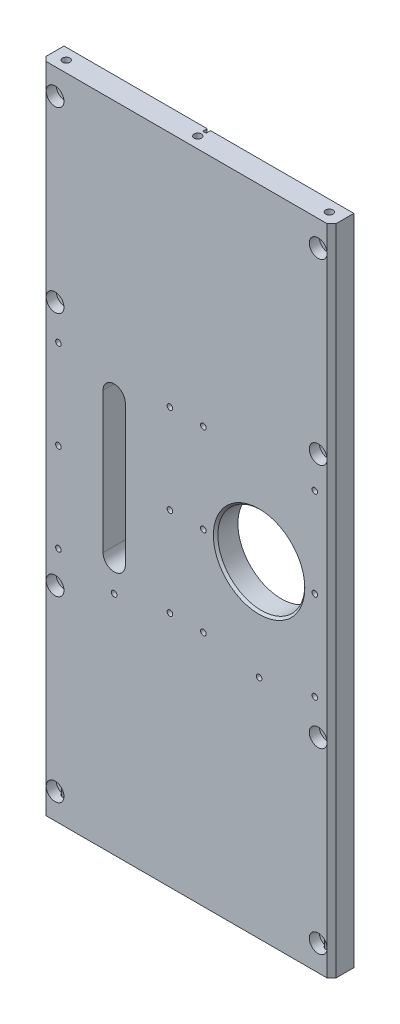
from build123d import *

# Parameters (mm, degrees)
SKETCH1_W                                            = 130
SKETCH1_H                                            = 293
BOSS_EXTRUDE1_DEPTH                                  = 5
SKETCH2_R                                            = 19.5
CUT_EXTRUDE1_DEPTH                                   = 161.584090121
CUT_EXTRUDE2_DEPTH                                   = 10
CHAMFER1_SIZE                                        = 2
HOLE_SIZE_PER_SOCKET_HEAD_CAP_SCREW_TYPE_D           = 4.5
HOLE_SIZE_PER_SOCKET_HEAD_CAP_SCREW_TYPE_CBORE_D     = 8
HOLE_SIZE_PER_SOCKET_HEAD_CAP_SCREW_TYPE_CBORE_DEPTH = 4.5
M3_TAPPED_HOLE1_AT_2_COUNT                           = 2
M3_TAPPED_HOLE1_AT_2_PITCH                           = 50
M3_TAPPED_HOLE1_AT_3_COUNT                           = 2
M3_TAPPED_HOLE1_AT_3_PITCH                           = 40
M3_TAPPED_HOLE1_AT_4_COUNT                           = 2
M3_TAPPED_HOLE1_AT_4_PITCH                           = 64.031242374
M3_TAPPED_HOLE1_AT_5_COUNT                           = 2
M3_TAPPED_HOLE1_AT_5_PITCH                           = 94.339811321
M3_TAPPED_HOLE1_AT_6_COUNT                           = 2
M3_TAPPED_HOLE1_AT_6_PITCH                           = 80
M3_TAPPED_HOLE2_D                                    = 2.5
M3_TAPPED_HOLE2_DEPTH                                = 8.5
M3_TAPPED_HOLE2_TIP                                  = 0.751075774
M4_TAPPED_HOLE1_AT_2_COUNT                           = 2
M4_TAPPED_HOLE1_AT_2_PITCH                           = 59
M4_TAPPED_HOLE1_AT_3_COUNT                           = 2
M4_TAPPED_HOLE1_AT_3_PITCH                           = 59
SKETCH12_W                                           = 1.5
SKETCH12_H                                           = 4
CUT_EXTRUDE3_DEPTH                                   = 301.164954749
M3_TAPPED_HOLE3_D                                    = 2.5
M3_TAPPED_HOLE3_DEPTH                                = 8.5
M3_TAPPED_HOLE3_TIP                                  = 0.751075774
CHAMFER2_SIZE                                        = 1


with BuildPart() as part:
    # Sketch1 → Boss-Extrude1 (new, symmetric)
    with BuildSketch(Plane.XY):
        Rectangle(SKETCH1_W, SKETCH1_H)
    extrude(amount=BOSS_EXTRUDE1_DEPTH, both=True)

    # Sketch2 → Cut-Extrude1 (cut, through all)
    with BuildSketch(Plane.XY.offset(5)):
        with Locations((32.5, 0)):
            Circle(SKETCH2_R)
    extrude(amount=-CUT_EXTRUDE1_DEPTH, mode=Mode.SUBTRACT)

    # Sketch3 → Cut-Extrude2 (cut)
    with BuildSketch(Plane.XY.offset(5)):
        with BuildLine():
            Line((-37.5, -31.5), (-37.5, 31.5))
            ThreePointArc((-37.5, 31.5), (-32.5, 36.5), (-27.5, 31.5))
            Line((-27.5, 31.5), (-27.5, -31.5))
            ThreePointArc((-27.5, -31.5), (-32.5, -36.5), (-37.5, -31.5))
        make_face()
    extrude(amount=-CUT_EXTRUDE2_DEPTH, mode=Mode.SUBTRACT)

    # Chamfer1
    chamfer1_edges = [part.edges().sort_by_distance(p)[0] for p in [
        (65, 0, 5),
        (-65, 0, 5),
    ]]
    chamfer(chamfer1_edges, length=CHAMFER1_SIZE)

    # Hole size per socket head cap screw type 1 (through all)
    with Locations(Plane.XY.offset(5)):
        with Locations((59, -135), (-59, -135), (59, -55), (-59, -55)):
            hole_size_per_socket_head_cap_screw_type = CounterBoreHole(HOLE_SIZE_PER_SOCKET_HEAD_CAP_SCREW_TYPE_D / 2, HOLE_SIZE_PER_SOCKET_HEAD_CAP_SCREW_TYPE_CBORE_D / 2, HOLE_SIZE_PER_SOCKET_HEAD_CAP_SCREW_TYPE_CBORE_DEPTH)

    # Mirror1: Hole size per socket head cap screw type 1 across plane
    add(hole_size_per_socket_head_cap_screw_type.mirror(Plane.ZX), mode=Mode.SUBTRACT)

    # Sketch6 → M3 Tapped Hole1 (revolve, cut)
    with BuildSketch(Plane(origin=(-7.5, -40, 5), x_dir=(0, -1, 0), z_dir=(1, 0, 0))):
        Polygon((0, 0), (0, 9.251075774), (1.25, 8.5), (1.25, 0), align=None)
    m3_tapped_hole1 = revolve(axis=Axis((-7.5, -40, 11.35), (0, 0, -1)), mode=Mode.SUBTRACT)

    # M3 Tapped Hole1 at 2: M3 Tapped Hole1 ×2
    with Locations(*[(-i * M3_TAPPED_HOLE1_AT_2_PITCH, 0, 0) for i in range(1, M3_TAPPED_HOLE1_AT_2_COUNT)]):
        add(m3_tapped_hole1, mode=Mode.SUBTRACT)

    # M3 Tapped Hole1 at 3: M3 Tapped Hole1 ×2
    with Locations(*[(0, i * M3_TAPPED_HOLE1_AT_3_PITCH, 0) for i in range(1, M3_TAPPED_HOLE1_AT_3_COUNT)]):
        add(m3_tapped_hole1, mode=Mode.SUBTRACT)

    # M3 Tapped Hole1 at 4: M3 Tapped Hole1 ×2
    with Locations(*[Vector(-0.7808688094430304, 0.6246950475544243, 0) * (i * M3_TAPPED_HOLE1_AT_4_PITCH) for i in range(1, M3_TAPPED_HOLE1_AT_4_COUNT)]):
        add(m3_tapped_hole1, mode=Mode.SUBTRACT)

    # M3 Tapped Hole1 at 5: M3 Tapped Hole1 ×2
    with Locations(*[Vector(-0.52999894000318, 0.847998304005088, 0) * (i * M3_TAPPED_HOLE1_AT_5_PITCH) for i in range(1, M3_TAPPED_HOLE1_AT_5_COUNT)]):
        add(m3_tapped_hole1, mode=Mode.SUBTRACT)

    # M3 Tapped Hole1 at 6: M3 Tapped Hole1 ×2
    with Locations(*[(0, i * M3_TAPPED_HOLE1_AT_6_PITCH, 0) for i in range(1, M3_TAPPED_HOLE1_AT_6_COUNT)]):
        add(m3_tapped_hole1, mode=Mode.SUBTRACT)

    # Mirror2: M3 Tapped Hole1 across plane
    add(m3_tapped_hole1.mirror(Plane.ZX), mode=Mode.SUBTRACT)

    # Mirror2 copy 1 sketch → Mirror2 copy 1 (revolve, cut)
    with BuildSketch(Plane(origin=(-57.5, 40, 5), x_dir=(0, 1, 0), z_dir=(1, 0, 0))):
        Polygon((0, 0), (0, -9.251075774), (1.25, -8.5), (1.25, 0), align=None)
    revolve(axis=Axis((-57.5, 40, 11.35), (0, 0, 1)), mode=Mode.SUBTRACT)

    # Mirror2 copy 2 sketch → Mirror2 copy 2 (revolve, cut)
    with BuildSketch(Plane(origin=(-7.5, 0, 5), x_dir=(0, 1, 0), z_dir=(1, 0, 0))):
        Polygon((0, 0), (0, -9.251075774), (1.25, -8.5), (1.25, 0), align=None)
    revolve(axis=Axis((-7.5, 0, 11.35), (0, 0, 1)), mode=Mode.SUBTRACT)

    # Mirror2 copy 3 sketch → Mirror2 copy 3 (revolve, cut)
    with BuildSketch(Plane(origin=(-57.5, 0, 5), x_dir=(0, 1, 0), z_dir=(1, 0, 0))):
        Polygon((0, 0), (0, -9.251075774), (1.25, -8.5), (1.25, 0), align=None)
    revolve(axis=Axis((-57.5, 0, 11.35), (0, 0, 1)), mode=Mode.SUBTRACT)

    # Mirror2 copy 4 sketch → Mirror2 copy 4 (revolve, cut)
    with BuildSketch(Plane(origin=(-57.5, -40, 5), x_dir=(0, 1, 0), z_dir=(1, 0, 0))):
        Polygon((0, 0), (0, -9.251075774), (1.25, -8.5), (1.25, 0), align=None)
    revolve(axis=Axis((-57.5, -40, 11.35), (0, 0, 1)), mode=Mode.SUBTRACT)

    # Mirror2 copy 5 sketch → Mirror2 copy 5 (revolve, cut)
    with BuildSketch(Plane(origin=(-7.5, -40, 5), x_dir=(0, 1, 0), z_dir=(1, 0, 0))):
        Polygon((0, 0), (0, -9.251075774), (1.25, -8.5), (1.25, 0), align=None)
    revolve(axis=Axis((-7.5, -40, 11.35), (0, 0, 1)), mode=Mode.SUBTRACT)

    # Mirror3: M3 Tapped Hole1 across plane
    add(m3_tapped_hole1.mirror(Plane(origin=(0, 0, 0), x_dir=(0, 0, 1), z_dir=(1, 0, 0))), mode=Mode.SUBTRACT)

    # Mirror3 copy 1 sketch → Mirror3 copy 1 (revolve, cut)
    with BuildSketch(Plane(origin=(57.5, -40, 5), x_dir=(0, -1, 0), z_dir=(-1, 0, 0))):
        Polygon((0, 0), (0, -9.251075774), (1.25, -8.5), (1.25, 0), align=None)
    revolve(axis=Axis((57.5, -40, 11.35), (0, 0, 1)), mode=Mode.SUBTRACT)

    # Mirror3 copy 2 sketch → Mirror3 copy 2 (revolve, cut)
    with BuildSketch(Plane(origin=(7.5, 0, 5), x_dir=(0, -1, 0), z_dir=(-1, 0, 0))):
        Polygon((0, 0), (0, -9.251075774), (1.25, -8.5), (1.25, 0), align=None)
    revolve(axis=Axis((7.5, 0, 11.35), (0, 0, 1)), mode=Mode.SUBTRACT)

    # Mirror3 copy 3 sketch → Mirror3 copy 3 (revolve, cut)
    with BuildSketch(Plane(origin=(57.5, 0, 5), x_dir=(0, -1, 0), z_dir=(-1, 0, 0))):
        Polygon((0, 0), (0, -9.251075774), (1.25, -8.5), (1.25, 0), align=None)
    revolve(axis=Axis((57.5, 0, 11.35), (0, 0, 1)), mode=Mode.SUBTRACT)

    # Mirror3 copy 4 sketch → Mirror3 copy 4 (revolve, cut)
    with BuildSketch(Plane(origin=(57.5, 40, 5), x_dir=(0, -1, 0), z_dir=(-1, 0, 0))):
        Polygon((0, 0), (0, -9.251075774), (1.25, -8.5), (1.25, 0), align=None)
    revolve(axis=Axis((57.5, 40, 11.35), (0, 0, 1)), mode=Mode.SUBTRACT)

    # Mirror3 copy 5 sketch → Mirror3 copy 5 (revolve, cut)
    with BuildSketch(Plane(origin=(7.5, 40, 5), x_dir=(0, -1, 0), z_dir=(-1, 0, 0))):
        Polygon((0, 0), (0, -9.251075774), (1.25, -8.5), (1.25, 0), align=None)
    revolve(axis=Axis((7.5, 40, 11.35), (0, 0, 1)), mode=Mode.SUBTRACT)

    # Mirror3 copy 6 sketch → Mirror3 copy 6 (revolve, cut)
    with BuildSketch(Plane(origin=(7.5, 40, 5), x_dir=(0, 1, 0), z_dir=(-1, 0, 0))):
        Polygon((0, 0), (0, 9.251075774), (1.25, 8.5), (1.25, 0), align=None)
    revolve(axis=Axis((7.5, 40, 11.35), (0, 0, -1)), mode=Mode.SUBTRACT)

    # Mirror3 copy 7 sketch → Mirror3 copy 7 (revolve, cut)
    with BuildSketch(Plane(origin=(57.5, 40, 5), x_dir=(0, 1, 0), z_dir=(-1, 0, 0))):
        Polygon((0, 0), (0, 9.251075774), (1.25, 8.5), (1.25, 0), align=None)
    revolve(axis=Axis((57.5, 40, 11.35), (0, 0, -1)), mode=Mode.SUBTRACT)

    # Mirror3 copy 8 sketch → Mirror3 copy 8 (revolve, cut)
    with BuildSketch(Plane(origin=(7.5, 0, 5), x_dir=(0, 1, 0), z_dir=(-1, 0, 0))):
        Polygon((0, 0), (0, 9.251075774), (1.25, 8.5), (1.25, 0), align=None)
    revolve(axis=Axis((7.5, 0, 11.35), (0, 0, -1)), mode=Mode.SUBTRACT)

    # Mirror3 copy 9 sketch → Mirror3 copy 9 (revolve, cut)
    with BuildSketch(Plane(origin=(57.5, 0, 5), x_dir=(0, 1, 0), z_dir=(-1, 0, 0))):
        Polygon((0, 0), (0, 9.251075774), (1.25, 8.5), (1.25, 0), align=None)
    revolve(axis=Axis((57.5, 0, 11.35), (0, 0, -1)), mode=Mode.SUBTRACT)

    # Mirror3 copy 10 sketch → Mirror3 copy 10 (revolve, cut)
    with BuildSketch(Plane(origin=(57.5, -40, 5), x_dir=(0, 1, 0), z_dir=(-1, 0, 0))):
        Polygon((0, 0), (0, 9.251075774), (1.25, 8.5), (1.25, 0), align=None)
    revolve(axis=Axis((57.5, -40, 11.35), (0, 0, -1)), mode=Mode.SUBTRACT)

    # Mirror3 copy 11 sketch → Mirror3 copy 11 (revolve, cut)
    with BuildSketch(Plane(origin=(7.5, -40, 5), x_dir=(0, 1, 0), z_dir=(-1, 0, 0))):
        Polygon((0, 0), (0, 9.251075774), (1.25, 8.5), (1.25, 0), align=None)
    revolve(axis=Axis((7.5, -40, 11.35), (0, 0, -1)), mode=Mode.SUBTRACT)

    # M3 Tapped Hole2
    with Locations(Plane(origin=(0, 0, -5), x_dir=(-1, 0, 0), z_dir=(0, 0, -1))):
        with Locations((-32.5, -139), (-32.5, 139)):
            Hole(M3_TAPPED_HOLE2_D / 2, depth=M3_TAPPED_HOLE2_DEPTH)
            with Locations((0, 0, -(M3_TAPPED_HOLE2_DEPTH + M3_TAPPED_HOLE2_TIP / 2))):  # 118° drill point
                Cone(0, M3_TAPPED_HOLE2_D / 2, M3_TAPPED_HOLE2_TIP, mode=Mode.SUBTRACT)

    # Sketch10 → M4 Tapped Hole1 (revolve, cut)
    with BuildSketch(Plane(origin=(0, -146.5, 0), x_dir=(0, 0, -1), z_dir=(1, 0, 0))):
        Polygon((0, 0), (0, 12.491420021), (1.65, 11.5), (1.65, 0), align=None)
    m4_tapped_hole1 = revolve(axis=Axis((0, -152.85, 0), (0, 1, 0)), mode=Mode.SUBTRACT)

    # M4 Tapped Hole1 at 2: M4 Tapped Hole1 ×2
    with Locations(*[(-i * M4_TAPPED_HOLE1_AT_2_PITCH, 0, 0) for i in range(1, M4_TAPPED_HOLE1_AT_2_COUNT)]):
        add(m4_tapped_hole1, mode=Mode.SUBTRACT)

    # M4 Tapped Hole1 at 3: M4 Tapped Hole1 ×2
    with Locations(*[(i * M4_TAPPED_HOLE1_AT_3_PITCH, 0, 0) for i in range(1, M4_TAPPED_HOLE1_AT_3_COUNT)]):
        add(m4_tapped_hole1, mode=Mode.SUBTRACT)

    # Mirror4: M4 Tapped Hole1 across plane
    add(m4_tapped_hole1.mirror(Plane.ZX), mode=Mode.SUBTRACT)

    # Mirror4 copy 1 sketch → Mirror4 copy 1 (revolve, cut)
    with BuildSketch(Plane(origin=(-59, 146.5, 0), x_dir=(0, 0, -1), z_dir=(1, 0, 0))):
        Polygon((0, 0), (0, -12.491420021), (1.65, -11.5), (1.65, 0), align=None)
    revolve(axis=Axis((-59, 152.85, 0), (0, 1, 0)), mode=Mode.SUBTRACT)

    # Mirror4 copy 2 sketch → Mirror4 copy 2 (revolve, cut)
    with BuildSketch(Plane(origin=(59, 146.5, 0), x_dir=(0, 0, -1), z_dir=(1, 0, 0))):
        Polygon((0, 0), (0, -12.491420021), (1.65, -11.5), (1.65, 0), align=None)
    revolve(axis=Axis((59, 152.85, 0), (0, 1, 0)), mode=Mode.SUBTRACT)

    # Sketch12 → Cut-Extrude3 (cut, through all)
    with BuildSketch(Plane(origin=(0, 146.5, 0), x_dir=(1, 0, 0), z_dir=(0, 1, 0))):
        with Locations((0, 5)):
            Rectangle(SKETCH12_W, SKETCH12_H)
    extrude(amount=-CUT_EXTRUDE3_DEPTH, mode=Mode.SUBTRACT)

    # M3 Tapped Hole3
    with Locations(Plane.XY.offset(5)):
        with Locations((-32.5, -45), (32.5, -45)):
            Hole(M3_TAPPED_HOLE3_D / 2, depth=M3_TAPPED_HOLE3_DEPTH)
            with Locations((0, 0, -(M3_TAPPED_HOLE3_DEPTH + M3_TAPPED_HOLE3_TIP / 2))):  # 118° drill point
                Cone(0, M3_TAPPED_HOLE3_D / 2, M3_TAPPED_HOLE3_TIP, mode=Mode.SUBTRACT)

    # Chamfer2
    chamfer2_edges = [part.edges().sort_by_distance(p)[0] for p in [
        (13, 0, 5),
    ]]
    chamfer(chamfer2_edges, length=CHAMFER2_SIZE)


solid = part.part
